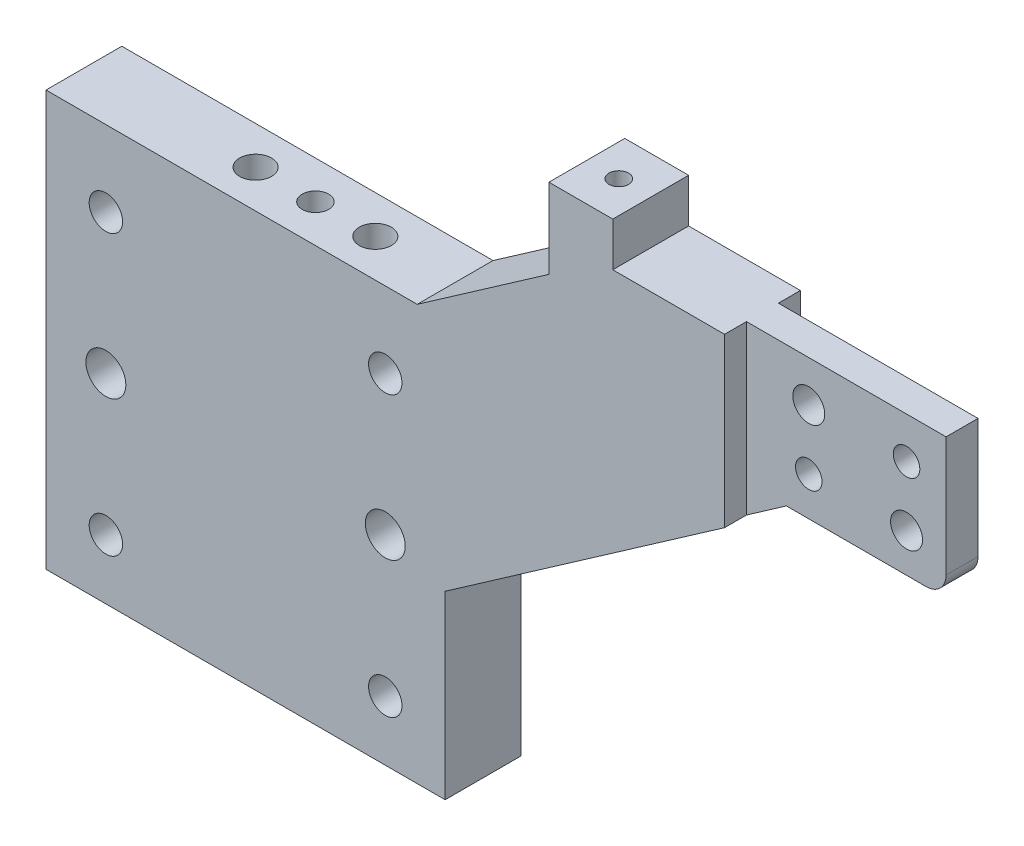
SolidWorks part; units mm, degrees
ref_plane "Front Plane" through (0, 0, 0) normal (0, 0, 1) x (1, 0, 0)
ref_plane "Top Plane" through (0, 0, 0) normal (0, 1, 0) x (1, 0, 0)
ref_plane "Right Plane" through (0, 0, 0) normal (1, 0, 0) x (0, 0, -1)
sketch "Sketch1" plane through (0, 0, 0) normal (0, 0, 1) x (1, 0, 0)
  line L0 (0, 0) -> (0, 104.0003)
  line L1 (0, 104.0003) -> (93, 104.0003)
  line L2 (93, 104.0003) -> (126, 127.0003)
  line L3 (126, 127.0003) -> (126, 147.0003)
  line L4 (126, 147.0003) -> (142, 147.0003)
  line L5 (142, 147.0003) -> (142, 136.0003)
  line L6 (142, 136.0003) -> (220, 136.0003)
  line L7 (220, 136.0003) -> (220, 101.0003)
  line L8 (220, 101.0003) -> (180, 101.0003)
  line L9 (180, 101.0003) -> (100, 45.2427)
  line L10 (100, 45.2427) -> (100, 0)
  line L11 (100, 0) -> (0, 0)
  line L12 (15, -11.693) -> (15, 133.0241) construction
  line L13 (85, 127.0003) -> (85, -6.7664) construction
  line L14 (-10.834, 15) -> (152.9735, 15) construction
  line L15 (-8.9865, 50) -> (158.2079, 50) construction
  line L16 (-16.6843, 85) -> (131.4199, 85) construction
  line L17 (165.2388, 110.7003) -> (233.0977, 110.7003) construction
  line L18 (161.6811, 125.7003) -> (232.3071, 125.7003) construction
  line L19 (210.1, 153.6884) -> (210.1, 87.6742) construction
  line L20 (185.6, 153.6884) -> (185.6, 93.4719) construction
  circle A0 centre (15, 15) radius 4.188
  circle A1 centre (15, 50) radius 5
  circle A2 centre (15, 85) radius 4.188
  circle A3 centre (85, 85) radius 4.188
  circle A4 centre (85, 50) radius 5
  circle A5 centre (85, 15) radius 4.188
  circle A6 centre (210.1, 125.7003) radius 3.3235
  circle A7 centre (210.1, 110.7003) radius 4
  circle A8 centre (185.6, 110.7003) radius 3.3235
  circle A9 centre (185.6, 125.7003) radius 4
  dimension "D17" = 9.9
  dimension "D1" = 104.0003
  dimension "D2" = 100
  dimension "D3" = 45.2427
  dimension "D4" = 93
  dimension "D5" = 23
  dimension "D6" = 33
  dimension "D7" = 20
  dimension "D8" = 16
  dimension "D9" = 11
  dimension "D10" = 78
  dimension "D11" = 97.5136
  dimension "D12" = 15
  dimension "D13" = 15
  dimension "D14" = 35
  dimension "D15" = 35
  dimension "D16" = 70
  dimension "D18" = 10.3
  dimension "D19" = 15
  dimension "D20" = 24.5
extrude "Boss-Extrude1" add sketch "Sketch1" along normal blind 19
ref_plane "Plane1" through (0, 104.0003, 0) normal (0, 1, 0) x (1, 0, 0)
sketch "Sketch2" plane through (0, 104.0003, 0) normal (0, 1, 0) x (1, 0, 0)
  line L0 (0, -9.5) -> (93, -9.5) construction
  line L1 (0, -19) -> (0, 0) construction
  line L2 (93, -19) -> (93, 0) construction
  circle A0 centre (43, -9.5) radius 4
  circle A1 centre (58, -9.5) radius 3.325
  circle A2 centre (73, -9.5) radius 4
  dimension "D1" = 43
  dimension "D2" = 15
  dimension "D3" = 15
extrude "Cut-Extrude1" cut sketch "Sketch2" against normal blind 15
ref_plane "Plane2" through (0, 147.0003, 0) normal (0, 1, 0) x (1, 0, 0)
sketch "Sketch3" plane through (0, 147.0003, 0) normal (0, 1, 0) x (1, 0, 0)
  line L0 (126, -9.5) -> (142, -9.5) construction
  line L1 (126, -19) -> (126, 0) construction
  line L2 (142, -19) -> (142, 0) construction
  circle A0 centre (134, -9.5) radius 2.4585
extrude "Cut-Extrude2" cut sketch "Sketch3" against normal blind 15
ref_plane "Plane3" through (0, 0, 19) normal (0, 0, 1) x (1, 0, 0)
sketch "Sketch4" plane through (0, 0, 19) normal (0, 0, 1) x (1, 0, 0)
  line L0 (100, 45.2427) -> (180, 101.0003) construction
  line L5 (220, 136.0003) -> (170, 136.0003)
  line L6 (220, 136.0003) -> (220, 94.0306)
  line L7 (220, 94.0306) -> (170, 94.0306)
  line L8 (170, 136.0003) -> (170, 94.0306)
  dimension "D1" = 50
extrude "Cut-Extrude3" cut sketch "Sketch4" against normal blind 5.5
ref_plane "Plane4" through (0, 0, 0) normal (0, 0, -1) x (-1, 0, 0)
sketch "Sketch5" plane through (0, 0, 0) normal (0, 0, -1) x (-1, 0, 0)
  line L0 (-100, 45.2427) -> (-180, 101.0003) construction
  line L5 (-220, 136.0003) -> (-170, 136.0003)
  line L6 (-220, 136.0003) -> (-220, 94.0306)
  line L7 (-220, 94.0306) -> (-170, 94.0306)
  line L8 (-170, 136.0003) -> (-170, 94.0306)
  dimension "D1" = 50
extrude "Cut-Extrude4" cut sketch "Sketch5" against normal blind 5.5
fillet "Fillet1" radius 5 1 edges at (220, 101.0003, 9.5)
